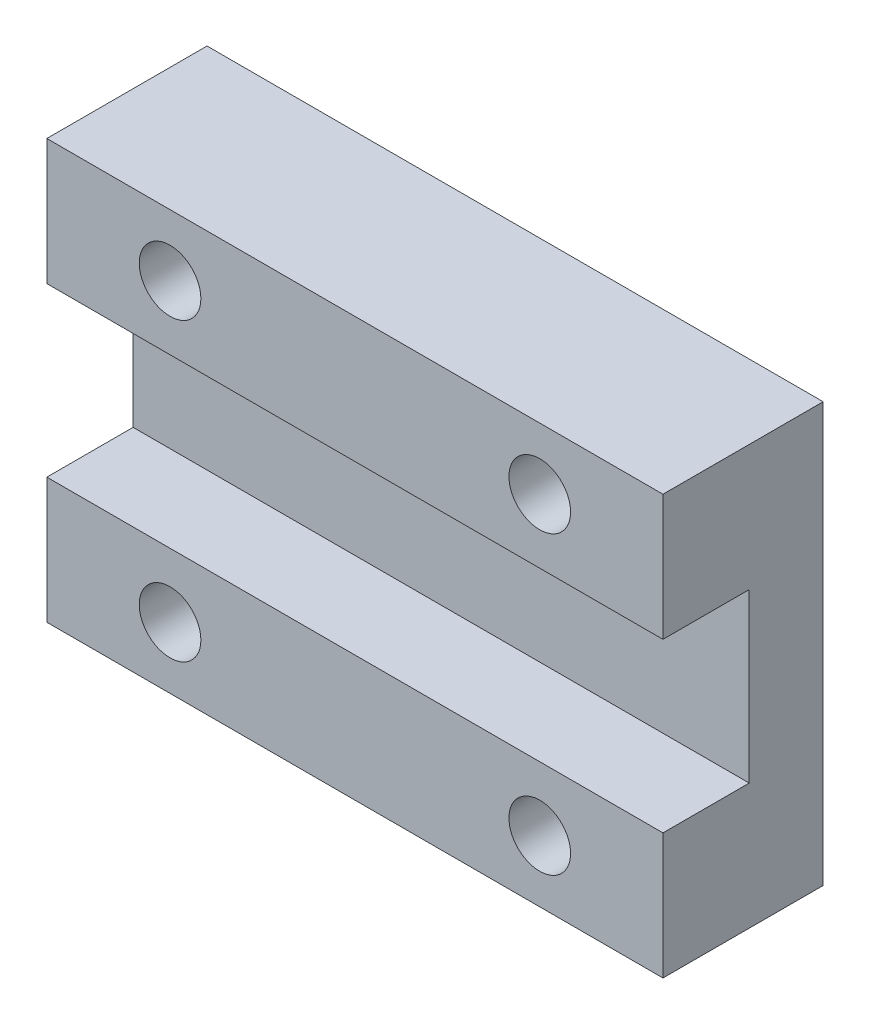
SolidWorks part; units mm, degrees
ref_plane "前视基准面" through (0, 0, 0) normal (0, 0, 1) x (1, 0, 0)
ref_plane "上视基准面" through (0, 0, 0) normal (0, 1, 0) x (1, 0, 0)
ref_plane "右视基准面" through (0, 0, 0) normal (1, 0, 0) x (0, 0, -1)
sketch "草图1" plane through (0, 0, 0) normal (0, 0, 1) x (1, 0, 0)
  line L1 (-13.0174, 11.5261) -> (11.9826, 11.5261)
  line L2 (-13.0174, 11.5261) -> (-13.0174, -5.4739)
  line L3 (-13.0174, -5.4739) -> (11.9826, -5.4739)
  line L4 (11.9826, 11.5261) -> (11.9826, -5.4739)
  dimension "D1" = 25
  dimension "D2" = 17
extrude "凸台-拉伸1" add sketch "草图1" along normal blind 6.5
sketch "草图2" plane through (11.9826, 0, 0) normal (1, 0, 0) x (0, 0, -1)
  line L0 (-6.5, -5.4739) -> (-6.5, 11.5261) construction
  line L1 (-6.5, -0.3739) -> (-3, -0.3739)
  line L2 (-6.5, -0.3739) -> (-6.5, 6.4261)
  line L3 (-6.5, 6.4261) -> (-3, 6.4261)
  line L4 (-3, -0.3739) -> (-3, 6.4261)
  line L5 (-6.5, 11.5261) -> (0, 11.5261) construction
  dimension "D1" = 6.8
  dimension "D2" = 3.5
  dimension "D3" = 5.1
extrude "切除-拉伸1" cut sketch "草图2" against normal up to next
sketch "草图3" plane through (0, 0, 6.5) normal (0, 0, 1) x (1, 0, 0)
  line L0 (11.9826, 11.5261) -> (-13.0174, 11.5261) construction
  line L1 (-13.0174, 11.5261) -> (-13.0174, 6.4261) construction
  circle A0 centre (-8.0174, 9.0261) radius 1.25
  circle A1 centre (6.9826, 9.0261) radius 1.25
  circle A2 centre (-8.0174, -2.9739) radius 1.25
  circle A3 centre (6.9826, -2.9739) radius 1.25
  dimension "D1" = 2.5
  dimension "D2" = 2.5
  dimension "D3" = 5
  dimension "D4" = 2
  dimension "D5" = 2
extrude "切除-拉伸2" cut sketch "草图3" against normal up to next
